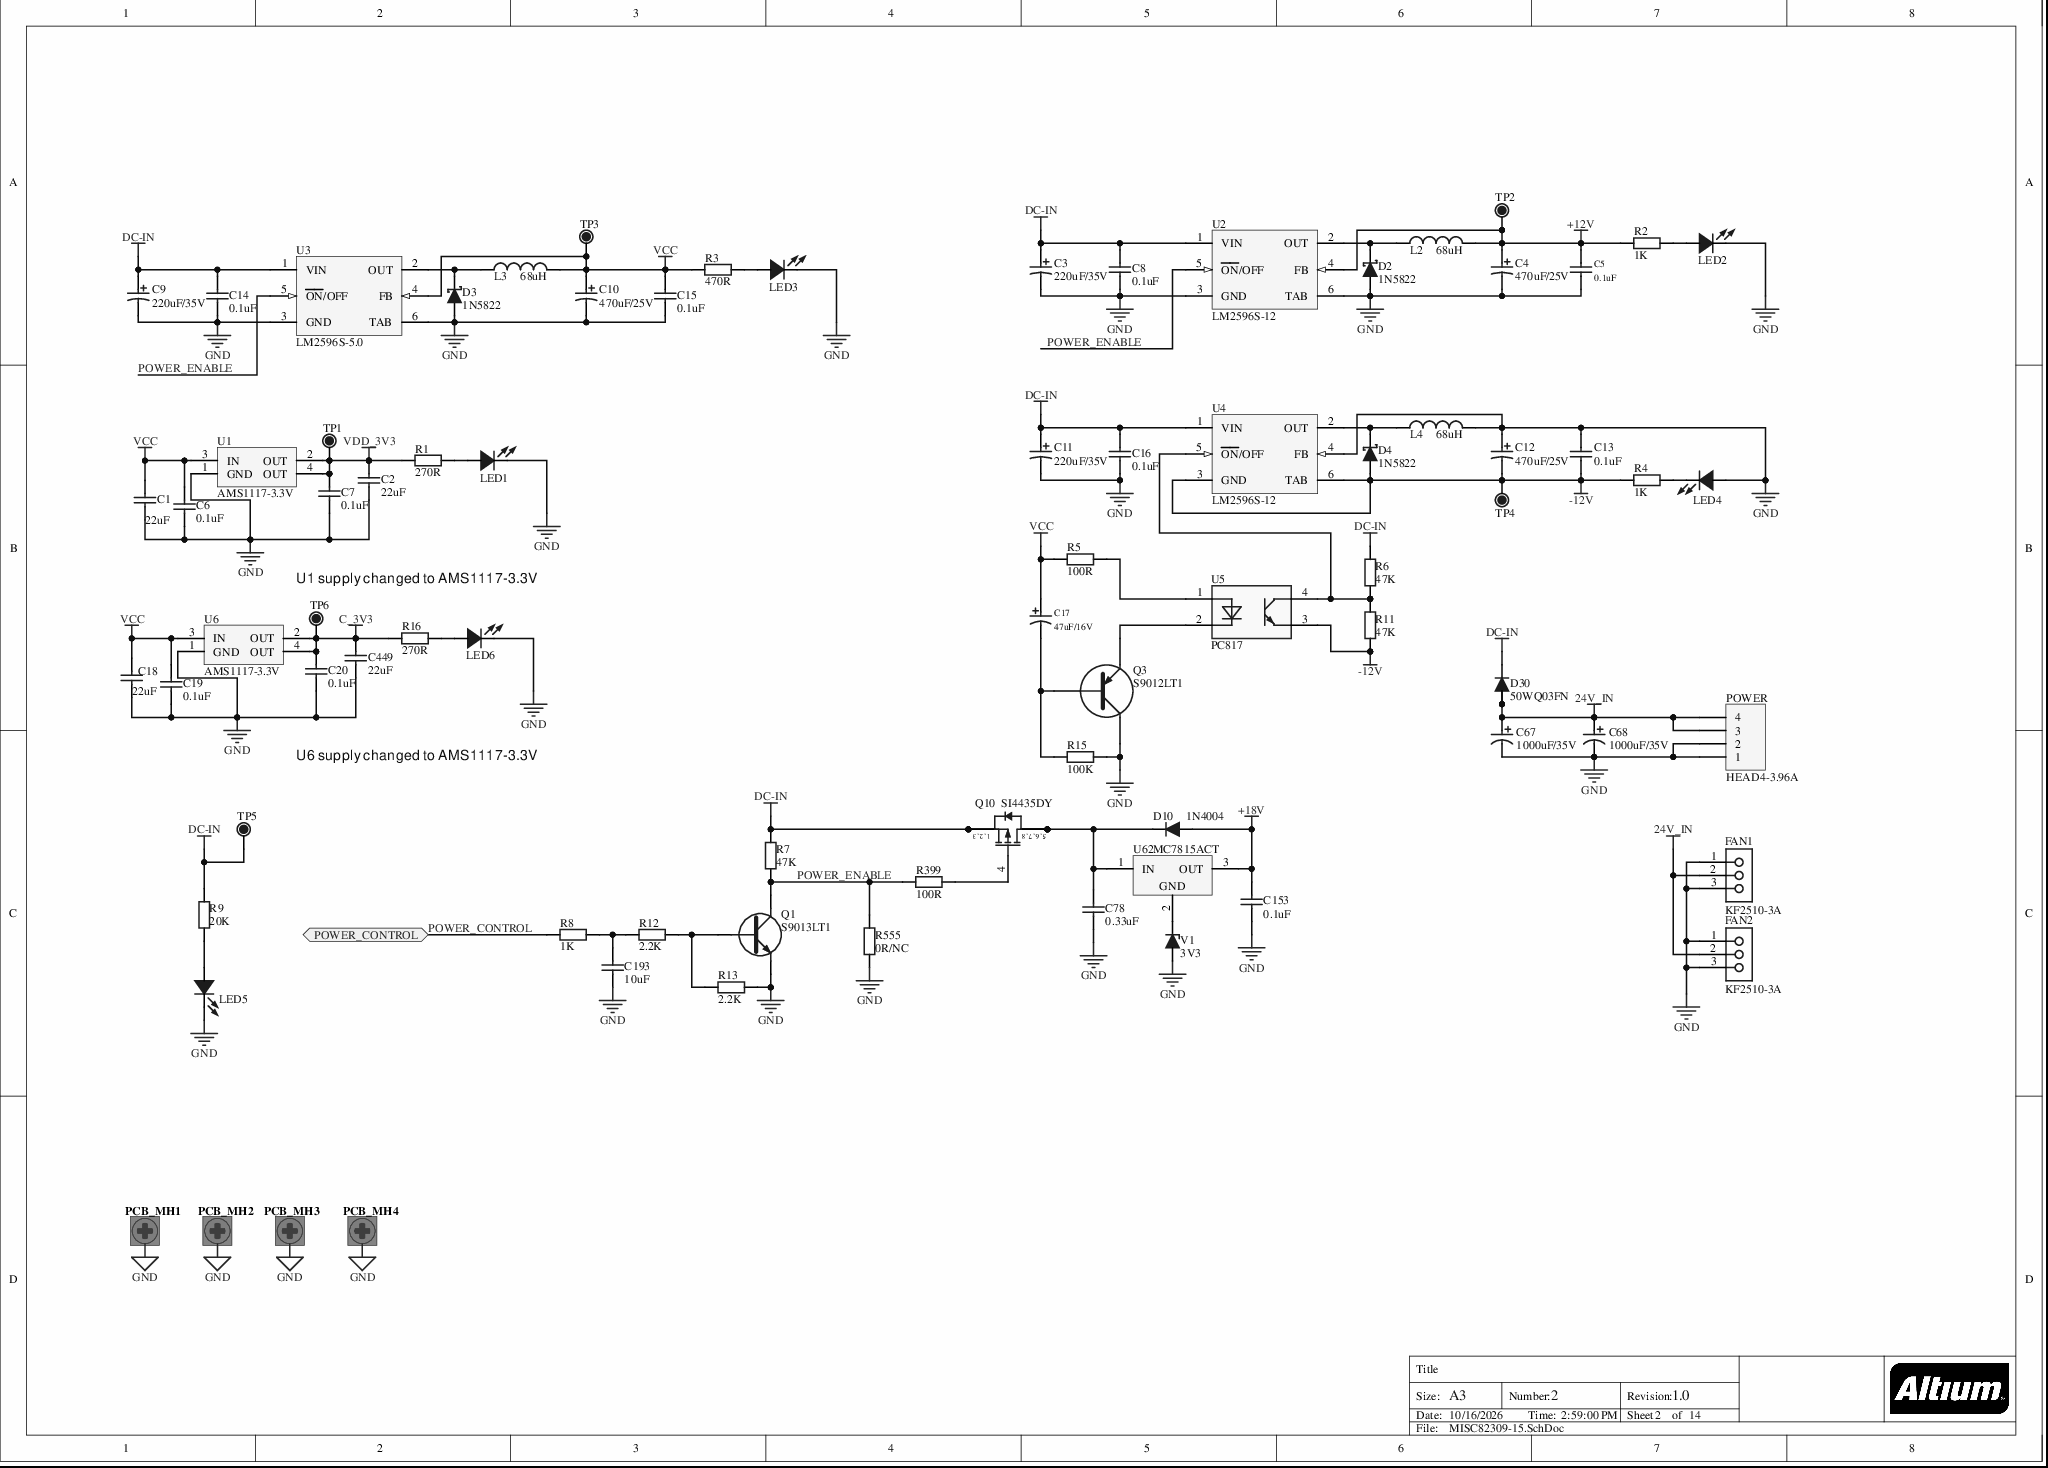
[diagram p0: MISC82309-15.SchDoc]
# Altium project MISC82309-16.PrjPcb (part 1 of 6)
13 sheets, 747 parts. Net scope: flat (ports and power ports of the same name join across sheets).
Board file: MISC82309.PcbDoc
Sheets:
  MISC82309-15.SchDoc
  MISC82309-11.SchDoc
  MISC82309-10.SchDoc
  MISC82309-8.SchDoc
  MISC82309-13.SchDoc
  MISC82309-12.SchDoc
  MISC82309-5.SchDoc
  MISC82309-6.SchDoc
  MISC82309-3.SchDoc
  MISC82309-4.SchDoc
  MISC82309-14.SchDoc
  MISC82309-9.SchDoc
  MISC82309-7.SchDoc

## Sheet MISC82309-15.SchDoc
size A3; DocumentNumber: 2; Revision: 1.0; SheetNumber: 2; SheetTotal: 14

### Parts
C1  22uF  [C0805]
C2  22uF  [C0805]
C3  220uF/35V  [E8X10,2]
C4  470uF/25V  [E10X10.2]
C5  0.1uF  [C1206]
C6  0.1uF  [C0603]
C7  0.1uF  [C0603]
C8  0.1uF  [C1206]
C9  220uF/35V  [E8X10,2]
C10  470uF/25V  [E10X10.2]
C11  220uF/35V  [E8X10,2]
C12  470uF/25V  [E10X10.2]
C13  0.1uF  [C1206]
C14  0.1uF  [C1206]
C15  0.1uF  [C1206]
C16  0.1uF  [C1206]
C17  47uF/16V  [E5X5.4]
C18  22uF  [C0805]
C19  0.1uF  [C0603]
C20  0.1uF  [C0603]
C67  1000uF/35V  [CAP-EL-12x20]
C68  1000uF/35V  [CAP-EL-12x20]
C78  0.33uF  [C1206]
C153  0.1uF  [C1206]
C193  10uF  [C0805]
C449  22uF  [C0805]
D2  1N5822  [D1810]
D3  1N5822  [D1810]
D4  1N5822  [D1810]
D10  1N4004  [DO-41 - 10.46mm]
D30  50WQ03FN  [TO-252AA]
FAN1  KF2510-3A  [KF2510-3A]
FAN2  KF2510-3A  [KF2510-3A]
L2  68uH  [L330]
L3  68uH  [L330]
L4  68uH  [L330]
LED1  LED  [LED_0805]  (value not drawn)
LED2  LED  [LED_0805]  (value not drawn)
LED3  LED  [LED_0805]  (value not drawn)
LED4  LED  [LED_0805]  (value not drawn)
LED5  LED  [LED_0805]  (value not drawn)
LED6  LED  [LED_0805]  (value not drawn)
PCB_MH1  MOUNTING HOLE 3MM  [MOUNTING_HOLE_3MM]  (value not drawn)  (no BOM)
PCB_MH2  MOUNTING HOLE 3MM  [MOUNTING_HOLE_3MM]  (value not drawn)  (no BOM)
PCB_MH3  MOUNTING HOLE 3MM  [MOUNTING_HOLE_3MM]  (value not drawn)  (no BOM)
PCB_MH4  MOUNTING HOLE 3MM  [MOUNTING_HOLE_3MM]  (value not drawn)  (no BOM)
POWER  HEAD4-3.96A  [VH-3_96-4]
Q1  S9013LT1  [SOT-23]
Q3  S9012LT1  [SOT-23]
Q10  SI4435DY  [SO-8_N]
R1  270R  [RES_0805]
R2  1K  [RES_0805]
R3  470R  [RES_0805]
R4  1K  [RES_0805]
R5  100R  [RES_0805]
R6  47K  [RES_0805]
R7  47K  [RES_0805]
R8  1K  [RES_0805]
R9  20K  [RES_0805]
R11  47K  [RES_0805]
R12  2.2K  [RES_0805]
R13  2.2K  [RES_0805]
R15  100K  [RES_0805]
R16  270R  [RES_0805]
R399  100R  [RES_0805]
R555  0R/NC  [RES_0603]
TP1  TP  [TPOINT]  (value not drawn)
TP2  TP  [TPOINT]  (value not drawn)
TP3  TP  [TPOINT]  (value not drawn)
TP4  TP  [TPOINT]  (value not drawn)
TP5  TP  [TPOINT]  (value not drawn)
TP6  TP  [TPOINT]  (value not drawn)
U1  AMS1117-3.3V  [SOT223]
U2  LM2596S-12  [TS5B_N]
U3  LM2596S-5.0  [TS5B_N]
U4  LM2596S-12  [TS5B_N]
U5  PC817  [SOIC_4N]
U6  AMS1117-3.3V  [SOT223]
U62  MC7815ACT  [TO220]
V1  3V3  [DO-213AA]

### Ports
POWER_CONTROL (bidir)

### Nets
24V_IN: C67.1 C68.1 D30.1 D30.3 FAN1.2 FAN2.2 POWER.3 POWER.4
+12V: C4.1 C5.1 L2.2 R2.1 TP2.1 U2.4(FB)
+18V: C153.1 D10.1 U62.3(OUT)
-12V: C12.2 C13.2 D4.1 R4.1 R11.1 TP4.1 U4.3(GND) U4.6(TAB) U5.3
C_3V3: C20.2 C449.2 R16.1 TP6.1 U6.2(OUT) U6.4(OUT)
DC-IN: C3.1 C8.2 C9.1 C11.1 C14.2 C16.2 D30.4 Q10.1(S) Q10.2(S) Q10.3(S) R6.2 R7.2 R9.2 TP5.1 U2.1(VIN) U3.1(VIN) U4.1(VIN)
GND: C1.1 C2.1 C3.2 C4.2 C5.2 C6.1 C7.1 C8.1 C9.2 C10.2 C11.2 C12.1 C13.1 C14.1 C15.2 C16.1 C18.1 C19.1 C20.1 C67.2 C68.2 C78.2 C153.2 C193.1 C449.1 D2.1 D3.1 FAN1.1 FAN1.3 FAN2.1 FAN2.3 L4.2 LED1.2(CATHODE) LED2.2(CATHODE) LED3.2(CATHODE) LED4.1(ANODE) LED5.2(CATHODE) LED6.2(CATHODE) POWER.1 POWER.2 Q1.2 Q3.3(C) R13.2 R15.2 R555.1 U1.1(GND) U2.3(GND) U2.6(TAB) U3.3(GND) U3.6(TAB) U4.4(FB) U6.1(GND) V1.1
VCC: C1.2 C6.2 C10.1 C15.1 C17.1 C18.2 C19.2 L3.2 R3.1 R5.1 TP3.1 U1.3(IN) U3.4(FB) U6.3(IN)
VDD_3V3: C2.2 C7.2 R1.1 TP1.1 U1.2(OUT) U1.4(OUT)
POWER_CONTROL: R8.1 ; port POWER_CONTROL
POWER_ENABLE: Q1.3 R7.1 R399.2 R555.2 U2.5(~{ON}/OFF) U3.5(~{ON}/OFF)
NetC17_2: C17.2 Q3.1(B) R15.1
NetC78_1: C78.1 D10.2 Q10.5(D) Q10.6(D) Q10.7(D) Q10.8(D) U62.1(IN)
NetC193_2: C193.2 R8.2 R12.1
NetD2_2: D2.2 L2.1 U2.2(OUT)
NetD3_2: D3.2 L3.1 U3.2(OUT)
NetD4_2: D4.2 L4.1 U4.2(OUT)
NetLED1_1: LED1.1(ANODE) R1.2
NetLED2_1: LED2.1(ANODE) R2.2
NetLED3_1: LED3.1(ANODE) R3.2
NetLED4_2: LED4.2(CATHODE) R4.2
NetLED5_1: LED5.1(ANODE) R9.1
NetLED6_1: LED6.1(ANODE) R16.2
NetQ1_1: Q1.1 R12.2 R13.1
NetQ3_2: Q3.2(E) U5.2
NetQ10_4: Q10.4(G) R399.1
NetR5_2: R5.2 U5.1
NetR6_1: R6.1 R11.2 U4.5(~{ON}/OFF) U5.4
NetU62_2: U62.2(GND) V1.2

Not connected (* = marked no-connect by the designer): PCB_MH1 0(GND) 1(GND) 2(GND) 3(GND) 4(GND) 5(GND) 6(GND) 7(GND) 8(GND) 9(GND) 10(GND); PCB_MH2 0(GND) 1(GND) 2(GND) 3(GND) 4(GND) 5(GND) 6(GND) 7(GND) 8(GND) 9(GND) 10(GND); PCB_MH3 0(GND) 1(GND) 2(GND) 3(GND) 4(GND) 5(GND) 6(GND) 7(GND) 8(GND) 9(GND) 10(GND); PCB_MH4 0(GND) 1(GND) 2(GND) 3(GND) 4(GND) 5(GND) 6(GND) 7(GND) 8(GND) 9(GND) 10(GND)

### Notes on the sheet
- U1 supply changed to AMS1117-3.3V
- U6 supply changed to AMS1117-3.3V
- Labels drawn without touching a wire or pin: GND
- Title
- Size:
- Date:
- A3
- Number:
- Time:
- Revision:
- Sheet
- of
- File:

### Library data of the parts
C1 C2 C6-C8 C14 C16 C19 C20 C193 = CAP_1206: Capacitor
  C1 C2: value: 22uF
  C6-C8 C14 C16 C19 C20: value: 0.1uF
  C193: value: 10uF
C3 C4 C9-C12 = CAP POL
  C3 C9 C11: value: 220uF/35V
  C4 C10 C12: value: 470uF/25V
C5 C13 C15 = CAP_0.1uF: value: 0.01uF
C17 = CAP_POLAR_1: Polar Capacitor
C18 C449 = CAP_1206: Capacitor; value: 10uF
C67 C68 = CAP_EL: Capacitor; value: 1000uF/35V
C78 = CAP_0.1uF: Capacitor 0.33uF; AEMS Code: 2100341; value: 0.33uF
C153 = CAP_0.1uF: Capacitor 0.1uF; AEMS Code: 2100341; value: 0.1uF
D10 = UF400X
L2-L4 = Inductor: value: 68uH
PCB_MH1-PCB_MH4 = MOUNTING_HOLE_3MM: Mounting Hole, M3 Screw, Plated, Square Pad; Category: Mounting-Hole; Status: Production
Q1 = Triode-NPN
Q3 = S9012LT1: PNP General  Purpose Transistors
Q10 = SI4435DY: P-Channel 30V (D-S) Rated  MOSFET; Published: 8-Jun-2000; LatestRevisionDate: 13-Apr-2006; LatestRevisionNote: IPC-7351 Footprint Added.; DatasheetVersion: 6-Oct-1997; PackageVersion: Aug-1998; PackageReference: SO-8; PackageDescription: 8-Pin Small Outline Integrated Circuit 1.27 mm Pitch; ComponentLink1Description: Manufacturer Link; ComponentLink1URL: http://www.vishay.com/; ComponentLink2Description: Datasheet; ComponentLink2URL: http://www.vishay.com/docs/70149/70149.pdf; Publisher: Altium Limited
R1-R9 R11-R13 R15 R16 R399 = Res_0805: Res
  R1 R16: value: 270R
  R2 R4 R8: value: 1K
  R3: value: 470R
  R5 R399: value: 100R
  R6 R7 R11: value: 47K
  R9: value: 20K
  R12 R13: value: 2.2K
  R15: value: 100K
R555 = Res_0603: Res; value: 0R/NC
TP1-TP6 = TP: Test Point; OriginalSymbolOrigin: (0,0)
U1 U6 = REG1117-3: 1A Low Dropout Positive Regulator Fixed; value: AMS1117-3.3V
U2 U4 = LM2596S-12: SIMPLE SWITCHER?Power Converter 150 KHz 3A Step-Down Voltage Regulator, 5-pin TO-263; Manufacturer: National Semiconductor; PackageTopMarking: NSUZXYTTE#*LM2596S*-12 P+; PowerWise: N; High-Reliability: Y; DatasheetVersion: May-2002; PackageVersion: revD, Apr-2005; PackageReference: TS5B; PackageDescription: TO-263, Molded, .400 x .390 x .180in, 5 Lead, .067in Pitch, Surface Mount; PartNumber: LM2596S-12; RoHS: N; PinCount: 5; CompType: Switcher; Code_JEDEC: MO-169-AB; ComponentLink1Description: Manufacturer URL; ComponentLink1URL: http://www.national.com/; ComponentLink2Description: LM2596 Datasheet; ComponentLink2URL: http://www.national.com/ds/LM/LM2596.pdf; ComponentLink3Description: LM2596 Web Page; ComponentLink3URL: http://www.national.com/pf/LM/LM2596.html; ComponentLink4Description: TS5B Package Page; ComponentLink4URL: http://www.national.com/packaging/folders/ts5b.html
U3 = LM2596S-5.0: SIMPLE SWITCHER?Power Converter 150 KHz 3A Step-Down Voltage Regulator, 5-pin TO-263; Manufacturer: National Semiconductor; PackageTopMarking: NSUZXYTTE#*LM2596S*-5.0 P+; PowerWise: N; High-Reliability: Y; DatasheetVersion: May-2002; PackageVersion: revD, Apr-2005; PackageReference: TS5B; PackageDescription: TO-263, Molded, .400 x .390 x .180in, 5 Lead, .067in Pitch, Surface Mount; PartNumber: LM2596S-5.0; RoHS: N; PinCount: 5; CompType: Switcher; Code_JEDEC: MO-169-AB; ComponentLink1Description: Manufacturer URL; ComponentLink1URL: http://www.national.com/; ComponentLink2Description: LM2596 Datasheet; ComponentLink2URL: http://www.national.com/ds/LM/LM2596.pdf; ComponentLink3Description: LM2596 Web Page; ComponentLink3URL: http://www.national.com/pf/LM/LM2596.html; ComponentLink4Description: TS5B Package Page; ComponentLink4URL: http://www.national.com/packaging/folders/ts5b.html
U62 = MC7815ACT: 3-Terminal Positive Fixed Voltage Regulator; Note: Pin 2 is electrically connected to TAB; Published: 17-Jul-2002; DatasheetVersion: 1988; PackageReference: 221A-04; PackageDescription: TO, Thru-Hole, Vertical, Heatsink Mounted; 3 In-Line Leads; Pitch 2.54 mm; Code_JEDEC: TO-262-AA; ComponentLink1Description: Manufacturer Link; ComponentLink1URL: http://www.onsemi.com/site/products/taxonomy/0,4438,503,00.html; ComponentLink2Description: Datasheet; ComponentLink2URL: http://www.onsemi.com/pub/Collateral/MC7800-D.PDF; Publisher: Altium Limited
V1 = Zener diode 3V3: Value: 3V3

## Sheet MISC82309-11.SchDoc
size A3; DocumentNumber: 3; Revision: 1.0; SheetNumber: 3; SheetTotal: 14
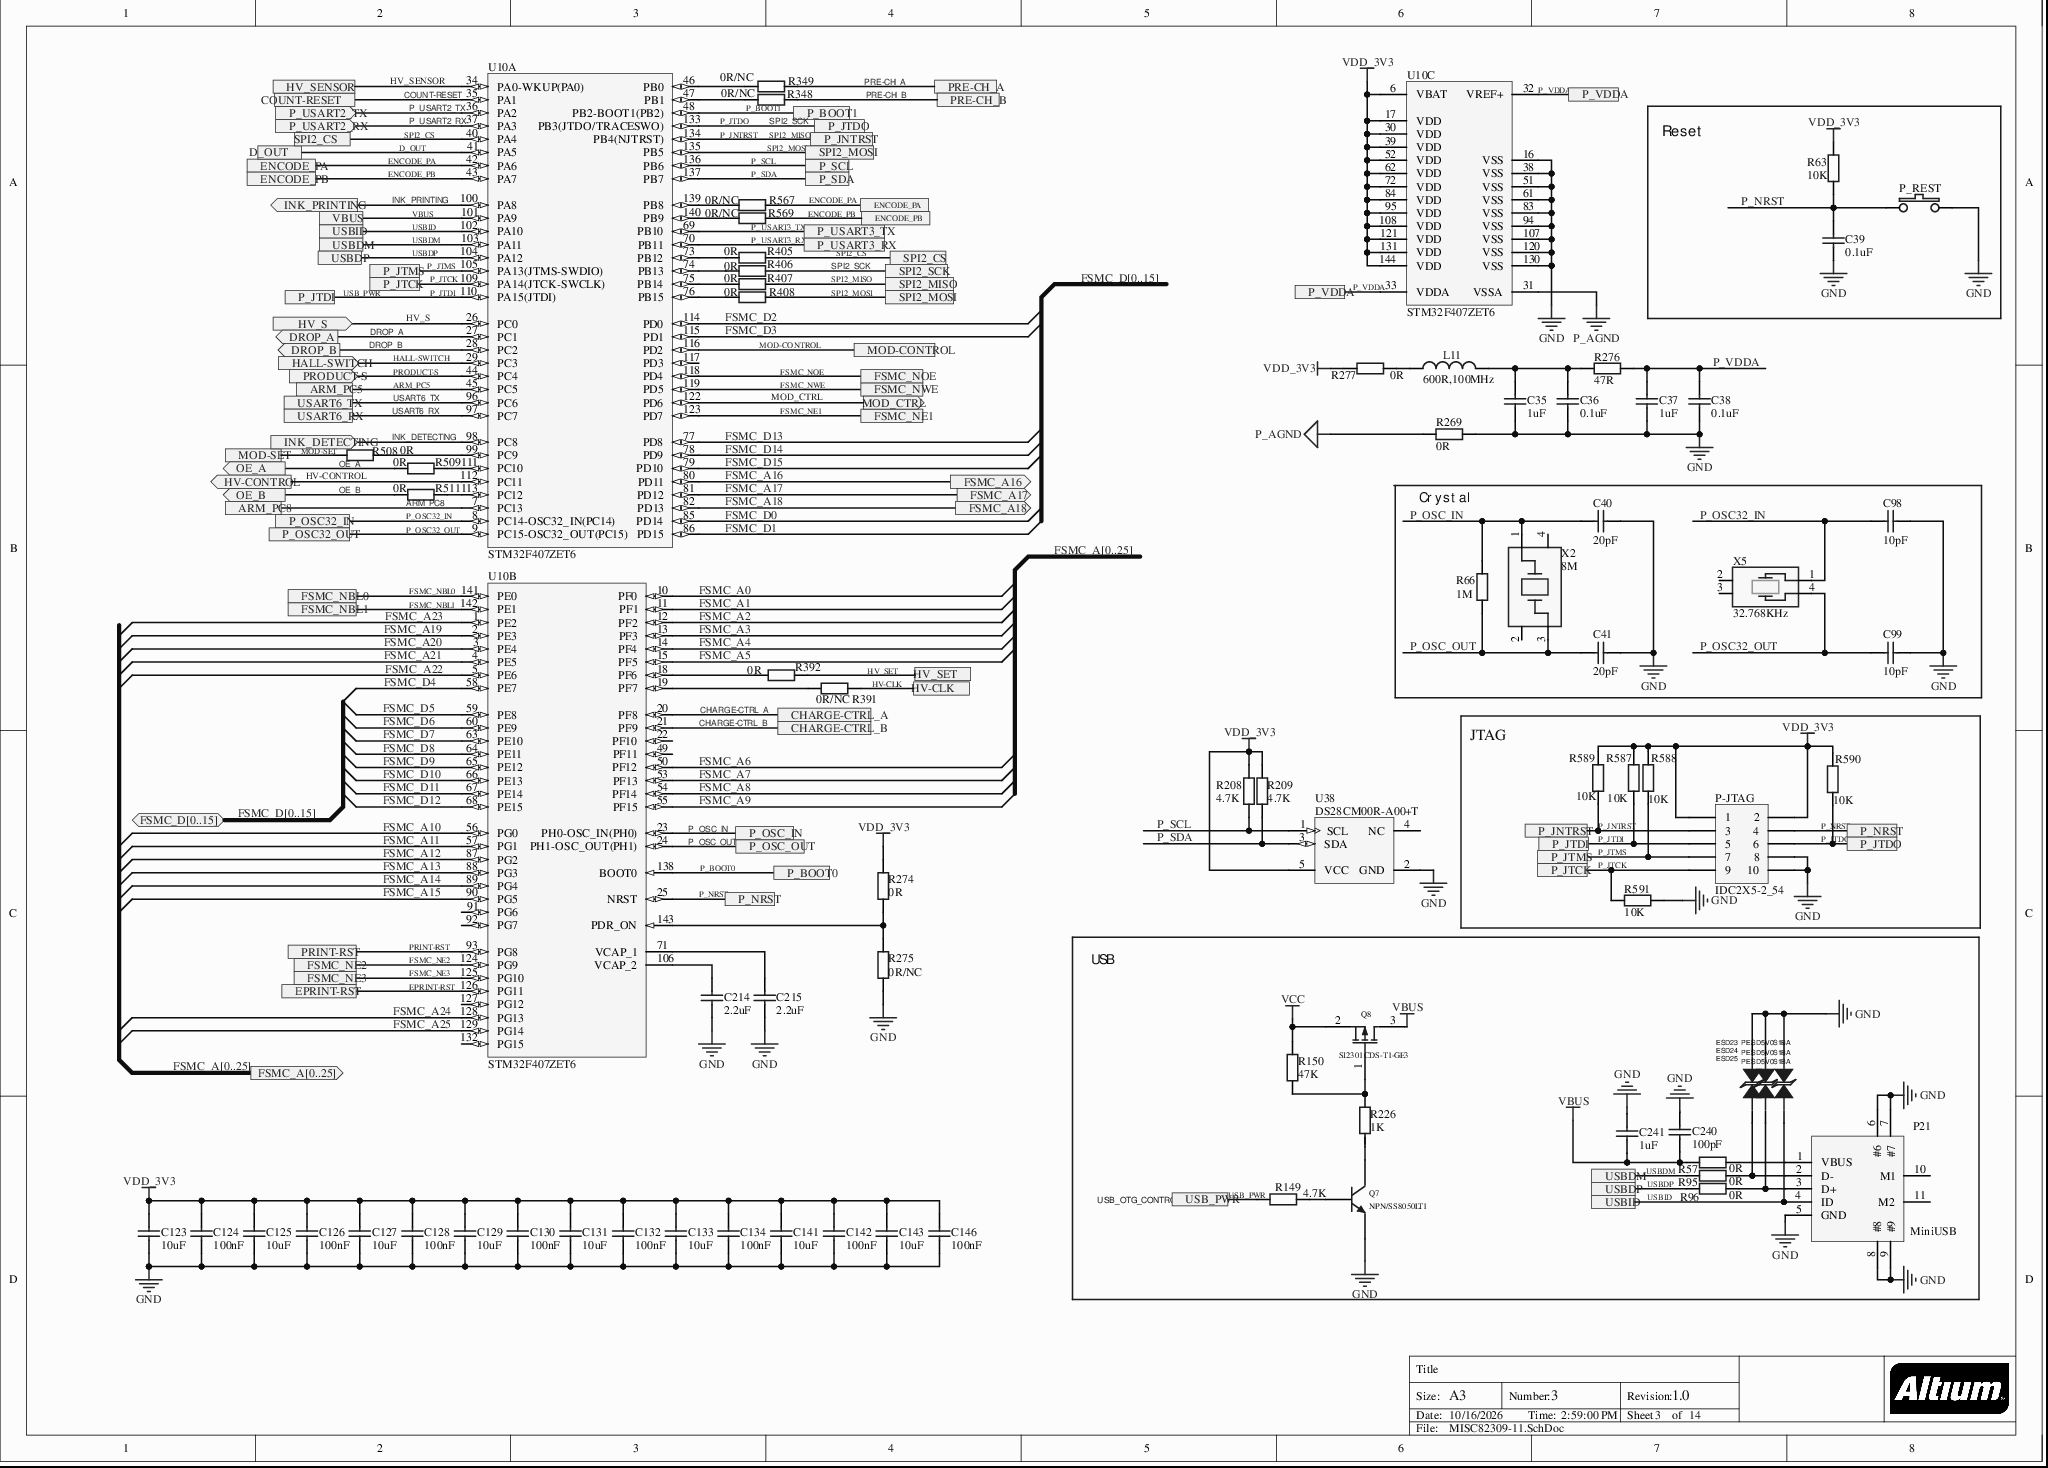
[diagram p1: MISC82309-11.SchDoc]

### Parts
C35  1uF  [CAP_0805]
C36  0.1uF  [CAP_0805]
C37  1uF  [CAP_0805]
C38  0.1uF  [CAP_0805]
C39  0.1uF  [C0603]
C40  20pF  [C0603]
C41  20pF  [C0603]
C98  10pF  [C0603]
C99  10pF  [C0603]
C123  10uF  [C0805]
C124  100nF  [C0805]
C125  10uF  [C0805]
C126  100nF  [C0805]
C127  10uF  [C0805]
C128  100nF  [C0805]
C129  10uF  [C0805]
C130  100nF  [C0805]
C131  10uF  [C0805]
C132  100nF  [C0805]
C133  10uF  [C0805]
C134  100nF  [C0805]
C141  10uF  [C0805]
C142  100nF  [C0805]
C143  10uF  [C0805]
C146  100nF  [C0805]
C214  2.2uF  [CAP_0805]
C215  2.2uF  [CAP_0805]
C240  100pF  [C0603]
C241  1uF  [C0603]
ESD23  PESD5V0S1BA  [SOD323]
ESD24  PESD5V0S1BA  [SOD323]
ESD25  PESD5V0S1BA  [SOD323]
L11  600R,100MHz  [R0805]
P21  MiniUSB  [MiniUSB-A]
P-JTAG  IDC2X5-2_54  [IDC2X5-2_54]
P_REST  SW  [SW-6X3X2.5]  (value not drawn)
Q7  NPN/SS8050LT1  [SOT-23-3]
Q8  SI2301CDS-T1-GE3  [SOT-23]
R57  0R  [RES_0603]
R63  10K  [R0603]
R66  1M  [R0603]
R95  0R  [RES_0603]
R96  0R  [RES_0603]
R149  4.7K  [R0603]
R150  47K  [RES_0603]
R208  4.7K  [R0603]
R209  4.7K  [R0603]
R226  1K  [RES_0603]
R269  0R  [R0805]
R274  0R  [RES_0603]
R275  0R/NC  [RES_0603]
R276  47R  [R0805]
R277  0R  [R0805]
R348  0R/NC  [RES_0603]
R349  0R/NC  [RES_0603]
R391  0R/NC  [RES_0603]
R392  0R  [RES_0603]
R405  0R  [RES_0603]
R406  0R  [RES_0603]
R407  0R  [RES_0603]
R408  0R  [RES_0603]
R508  0R  [RES_0603]
R509  0R  [RES_0603]
R511  0R  [RES_0603]
R567  0R/NC  [RES_0603]
R569  0R/NC  [RES_0603]
R587  10K  [R0603]
R588  10K  [R0603]
R589  10K  [R0603]
R590  10K  [R0603]
R591  10K  [R0603]
U10  STM32F407ZET6  [LQFP144]  (parts A,B,C of 3)
U38  DS28CM00R-A00+T  [U5+1_N]
X2  8M  [SMD5032]
X5  32.768KHz  [Y_XTAL_T7]

### Blocks framed on the sheet
Reset: C39 P_REST R63
Crystal: C40 C41 C98 C99 R66 X2 X5
JTAG: P-JTAG R587-R591
USB: C240 C241 ESD23-ESD25 P21 Q7 Q8 R57 R95 R96 R149 R150 R226

### Ports
ARM_PC5, ARM_PC8, CHARGE-CTRL_A, CHARGE-CTRL_B, COUNT-RESET, D_OUT, DROP_A (out), DROP_B (out), ENCODE_PA, ENCODE_PB, EPRINT-RST, FSMC_A16 (out), FSMC_A17 (out), FSMC_A18 (out), FSMC_A[0..25] (out), FSMC_D[0..15] (bidir), FSMC_NBL0, FSMC_NBL1, FSMC_NE1, FSMC_NE2, FSMC_NE3, FSMC_NOE, FSMC_NWE, HALL-SWITCH (in), HV-CLK, HV-CONTROL (out), HV_S (in), HV_SENSOR, HV_SET, INK_DETECTING (in), INK_PRINTING (out), MOD-CONTROL, MOD-SET, MOD_CTRL (out), OE_A (out), OE_B (out), P_BOOT0, P_BOOT1, P_JNTRST, P_JTCK, P_JTDI, P_JTDO, P_JTMS, P_NRST, P_OSC32_IN, P_OSC32_OUT, P_OSC_IN, P_OSC_OUT, P_SCL, P_SDA, P_USART2_RX (in), P_USART2_TX (in), P_USART3_RX, P_USART3_TX, P_VDDA, PRE-CH_A, PRE-CH_B, PRINT-RST, PRODUCT-S (in), SPI2_CS, SPI2_MISO, SPI2_MOSI, SPI2_SCK, USART6_RX, USART6_TX, USB_PWR, USBDM, USBDP, USBID, VBUS

### Nets
GND: C35.1 C36.1 C37.1 C38.1 C39.1 C40.1 C41.1 C98.1 C99.1 C123.1 C124.1 C125.1 C126.1 C127.1 C128.1 C129.1 C130.1 C131.1 C132.1 C133.1 C134.1 C141.1 C142.1 C143.1 C146.1 C214.2 C215.2 C240.1 C241.1 ESD23.2 ESD24.2 ESD25.2 P21.5(GND) P21.6(#6) P21.7(#7) P21.8(#8) P21.9(#9) P-JTAG.8 P-JTAG.10 P_REST.2 Q7.2(E) R269.2 R275.1 R591.1 U10.16(VSS) U10.38(VSS) U10.51(VSS) U10.61(VSS) U10.83(VSS) U10.94(VSS) U10.107(VSS) U10.120(VSS) U10.130(VSS) U38.2(GND)
P_AGND: R269.1 U10.31(VSSA)
VBUS: C240.2 C241.2 Q8.3(D) R57.2 U10.101(PA9) ; port VBUS
VCC: Q8.2(S) R150.2
VDD_3V3: C123.2 C124.2 C125.2 C126.2 C127.2 C128.2 C129.2 C130.2 C131.2 C132.2 C133.2 C134.2 C141.2 C142.2 C143.2 C146.2 P-JTAG.1 P-JTAG.2 R63.1 R208.1 R209.1 R274.2 R277.1 R587.2 R588.2 R589.2 R590.2 U10.6(VBAT) U10.17(VDD) U10.30(VDD) U10.39(VDD) U10.52(VDD) U10.62(VDD) U10.72(VDD) U10.84(VDD) U10.95(VDD) U10.108(VDD) U10.121(VDD) U10.131(VDD) U10.144(VDD) U38.5(VCC)